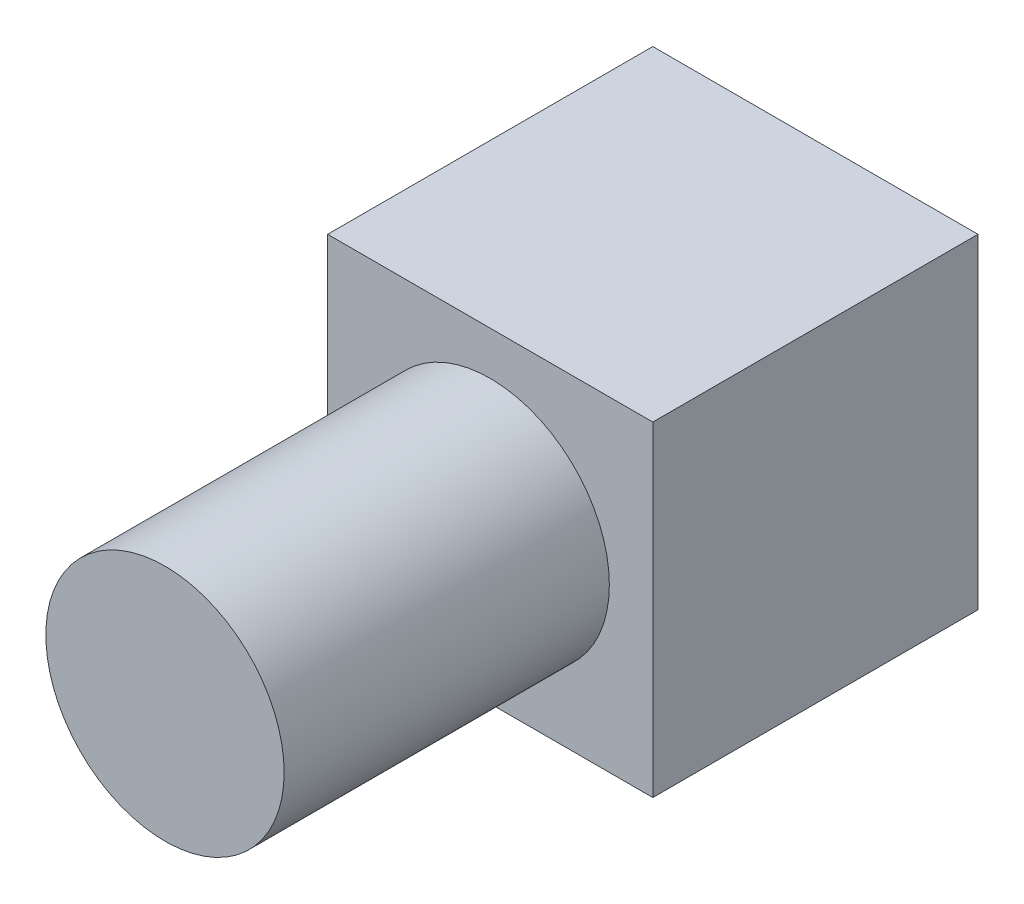
SolidWorks part; units mm, degrees
ref_plane "Front Plane" through (0, 0, 0) normal (0, 0, 1) x (1, 0, 0)
ref_plane "Top Plane" through (0, 0, 0) normal (0, 1, 0) x (1, 0, 0)
ref_plane "Right Plane" through (0, 0, 0) normal (1, 0, 0) x (0, 0, -1)
sketch "Sketch1" plane through (0, 0, 0) normal (0, 1, 0) x (1, 0, 0)
  line L1 (-30, 30) -> (30, 30)
  line L2 (-30, 30) -> (-30, -30)
  line L3 (-30, -30) -> (30, -30)
  line L4 (30, 30) -> (30, -30)
  line L5 (-30, 30) -> (30, -30) construction
  line L6 (-30, -30) -> (30, 30) construction
  point P0 (0, 0)
  dimension "D1" = 60
  dimension "D2" = 60
extrude "Boss-Extrude1" add sketch "Sketch1" along normal blind 60
sketch "Sketch2" plane through (0, 0, 30) normal (0, 0, 1) x (1, 0, 0)
  line L0 (-30, 60) -> (-30, 0) construction
  circle A0 centre (0, 30) radius 21.9848
  point P4 (-30, 30)
extrude "Boss-Extrude2" add sketch "Sketch2" along normal blind 60
